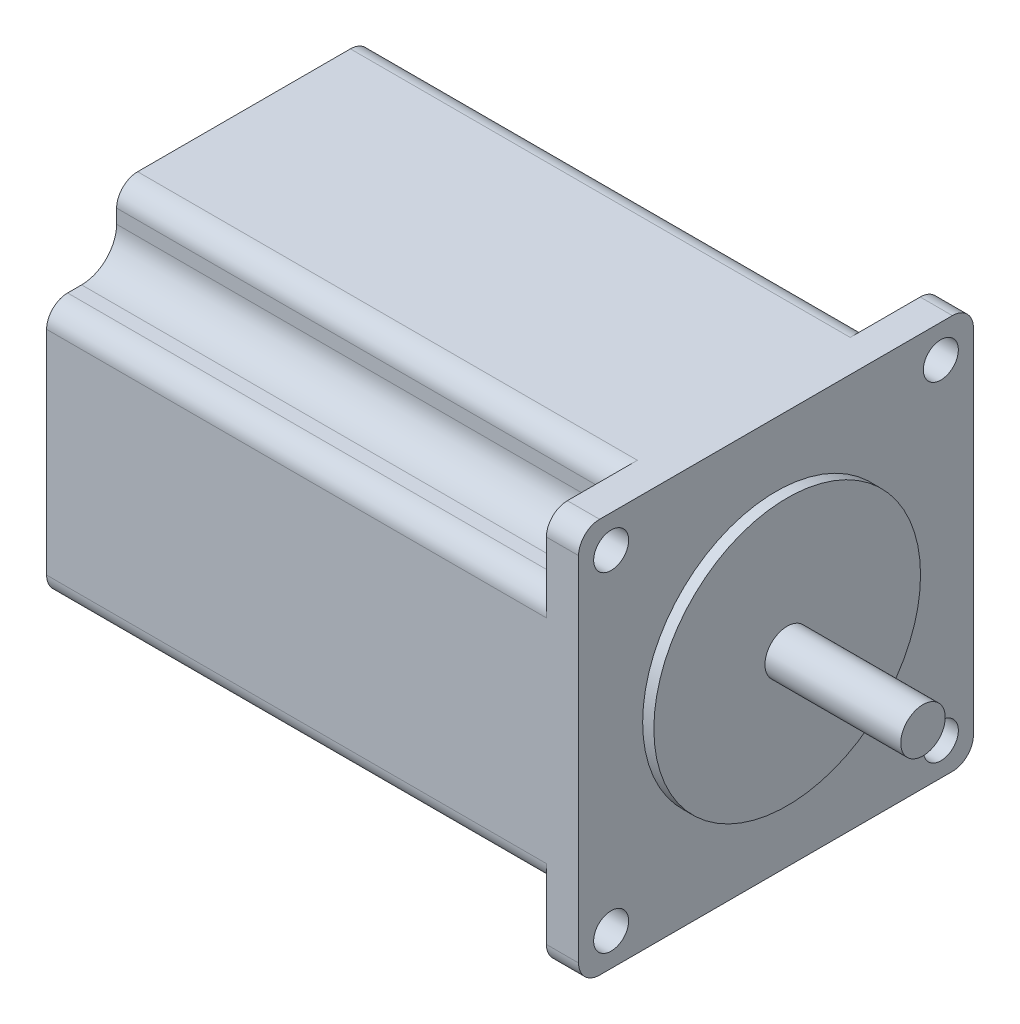
SolidWorks part; units mm, degrees
ref_plane "前视基准面" through (0, 0, 0) normal (0, 0, 1) x (1, 0, 0)
ref_plane "上视基准面" through (0, 0, 0) normal (0, 1, 0) x (1, 0, 0)
ref_plane "右视基准面" through (0, 0, 0) normal (1, 0, 0) x (0, 0, -1)
sketch "草图1" plane through (0, 0, 0) normal (1, 0, 0) x (0, 0, -1)
  line L1 (-28.2, -28.2) -> (28.2, -28.2)
  line L2 (-28.2, -28.2) -> (-28.2, 28.2)
  line L3 (-28.2, 28.2) -> (28.2, 28.2)
  line L4 (28.2, -28.2) -> (28.2, 28.2)
  line L5 (-28.2, -28.2) -> (28.2, 28.2) construction
  line L6 (-28.2, 28.2) -> (28.2, -28.2) construction
  point P0 (0, 0)
  dimension "D1" = 56.4
  dimension "D2" = 56.4
extrude "凸台-拉伸1" add sketch "草图1" along normal blind 76
sketch "草图2" plane through (76, 0, 0) normal (1, 0, 0) x (0, 0, -1)
  circle A0 centre (0, 0) radius 19.05
  dimension "D1" = 38.1
extrude "凸台-拉伸2" add sketch "草图2" along normal blind 1.6
sketch "草图3" plane through (77.6, 0, 0) normal (1, 0, 0) x (0, 0, -1)
  circle A0 centre (0, 0) radius 3.175
  dimension "D1" = 6.35
extrude "凸台-拉伸3" add sketch "草图3" along normal blind 19.4
fillet "圆角1" radius 3 4 edges at (38, -28.2, -28.2) (38, -28.2, 28.2) (38, 28.2, -28.2) (38, 28.2, 28.2)
sketch "草图4" plane through (0, 0, 0) normal (-1, 0, 0) x (0, 0, 1)
  line L0 (-28.2, -25.2) -> (-28.2, 25.2) construction
  line L1 (-28.2, 28.2) -> (-18.2, 28.2)
  line L2 (-28.2, 28.2) -> (-28.2, 18.2)
  line L3 (-28.2, 18.2) -> (-23.2, 18.2)
  line L4 (-18.2, 28.2) -> (-18.2, 23.2)
  line L5 (-25.2, 28.2) -> (25.2, 28.2) construction
  arc A0 (-18.2, 23.2) -> (-23.2, 18.2) centre (-23.2, 23.2) cw
  dimension "D1" = 5
  dimension "D2" = 10
  dimension "D3" = 10
extrude "切除-拉伸1" cut sketch "草图4" against normal offset from surface (71.4 mm away) 4.6 up to face at (76, 0, 0)
sketch "草图5" plane through (71.4, 0, 0) normal (-1, 0, 0) x (0, 0, 1)
  line L0 (0, -28.2) -> (0, 33.6822) construction
  line L1 (25.2, -28.2) -> (-25.2, -28.2) construction
  line L2 (0, 0) -> (28.2, 0) construction
  line L3 (28.2, 25.2) -> (28.2, -25.2) construction
  circle A0 centre (-23.55, 23.55) radius 2.5
  dimension "D1" = 5
  dimension "D2" = 47.1
  dimension "D3" = 47.1
extrude "切除-拉伸2" cut sketch "草图5" against normal blind 5
pattern_circular "阵列(圆周)3" count 4 over 360 about axis through (0, 0, 0) along (1, 0, 0) of "切除-拉伸2", "切除-拉伸1"
fillet "圆角2" radius 3 8 edges at (35.7, 18.2, -28.2) (35.7, 28.2, -18.2) (35.7, 18.2, 28.2) (35.7, 28.2, 18.2) (35.7, -18.2, 28.2) (35.7, -28.2, 18.2) (35.7, -28.2, -18.2) (35.7, -18.2, -28.2)
